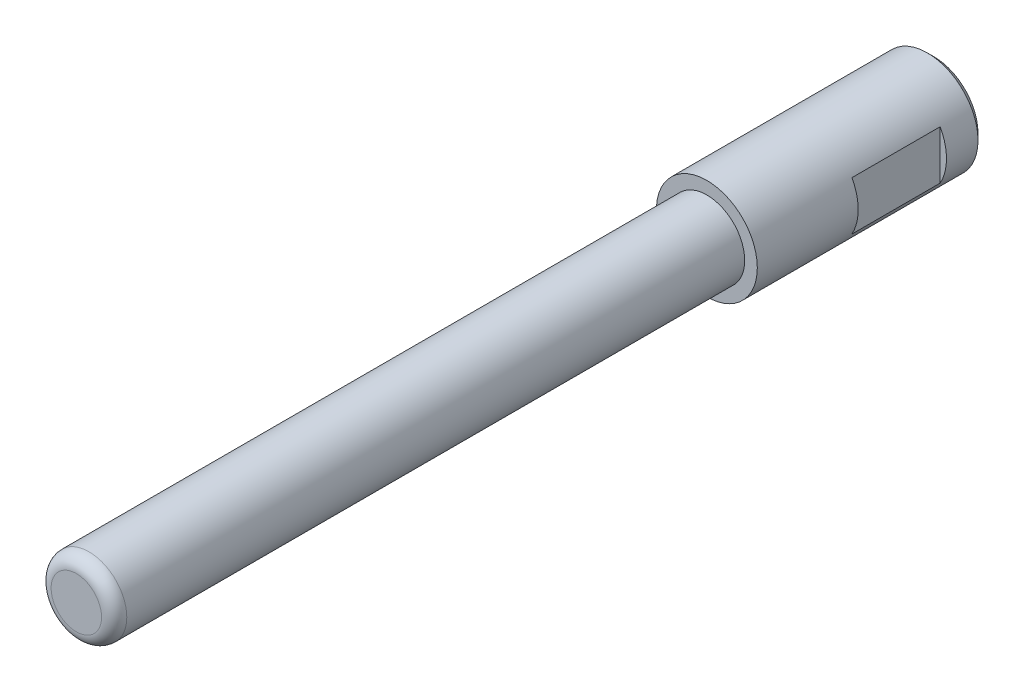
SolidWorks part; units mm, degrees
material "米黄色赛刚"
ref_plane "前视基准面" through (0, 0, 0) normal (0, 0, 1) x (1, 0, 0)
ref_plane "上视基准面" through (0, 0, 0) normal (0, 1, 0) x (1, 0, 0)
ref_plane "右视基准面" through (0, 0, 0) normal (1, 0, 0) x (0, 0, -1)
sketch "草图1" plane through (0, 0, 0) normal (0, 0, 1) x (1, 0, 0)
  circle A0 centre (0, 0) radius 4
  dimension "D1" = 8
extrude "凸台-拉伸1" add sketch "草图1" along normal blind 18
sketch "草图2" plane through (0, 0, 18) normal (0, 0, 1) x (1, 0, 0)
  circle A0 centre (0, 0) radius 3
  dimension "D1" = 6
extrude "凸台-拉伸2" add sketch "草图2" along normal blind 50
fillet "圆角1" radius 1 1 edges at (3, 0, 68)
chamfer "倒角1" distance 0.5 angle 45 1 edges at (4, 0, 0)
hole_wizard "M4 螺纹孔1" positions "草图4" profile "草图3" tap size "M4" standard "GB"
sketch "草图4" plane through (0, 0, 0) normal (0, 0, -1) x (-1, 0, 0)
  point P0 (0, 0)
sketch "草图3" plane through (0, 0, 0) normal (1, 0, 0) x (0, 1, 0)
  line L0 (0, 0) -> (0, 14.4914)
  line L1 (0, 14.4914) -> (1.65, 13.5)
  line L2 (1.65, 13.5) -> (1.65, 0)
  line L5 (1.65, 0) -> (0, 0)
  line L10 (0, 14.4914) -> (-1.65, 13.5) construction
  line L11 (0, -6.35) -> (0, 107.95) construction
  dimension "螺纹孔钻头直径" = 3.3
  dimension "螺纹孔钻头深度" = 13.5
  dimension "导头角度" = 118
cosmetic thread "孔螺蚊线1" parameters "D1"=10, "D2"=4
ref_plane "基准面1" through (0, 0, 3) normal (0, 0, -1) x (-1, 0, 0)
sketch "草图5" plane through (0, 0, 3) normal (0, 0, -1) x (-1, 0, 0)
  line L1 (-6.1009, 4.5453) -> (-3.5, 4.5453)
  line L2 (-6.1009, 4.5453) -> (-6.1009, -5.2141)
  line L3 (-6.1009, -5.2141) -> (-3.5, -5.2141)
  line L4 (-3.5, 4.5453) -> (-3.5, -5.2141)
  line L5 (3.5, 4.5453) -> (7.81, 4.5453)
  line L6 (3.5, 4.5453) -> (3.5, -5.0407)
  line L7 (3.5, -5.0407) -> (7.81, -5.0407)
  line L8 (7.81, 4.5453) -> (7.81, -5.0407)
  dimension "D1" = 3.5
  dimension "D2" = 3.5
extrude "切除-拉伸1" cut sketch "草图5" against normal blind 7
